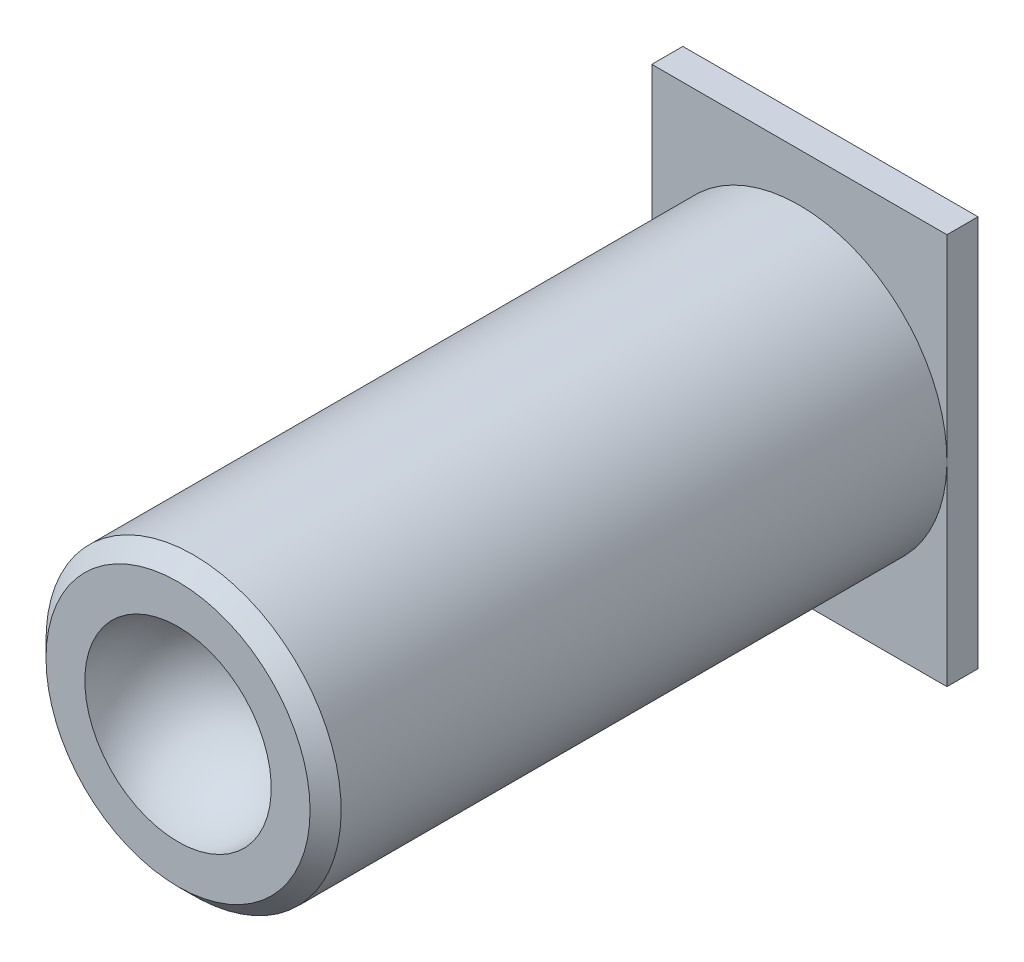
SolidWorks part; units mm, degrees
material "橡胶"
ref_plane "Front Plane" through (0, 0, 0) normal (0, 0, 1) x (1, 0, 0)
ref_plane "Top Plane" through (0, 0, 0) normal (0, 1, 0) x (1, 0, 0)
ref_plane "Right Plane" through (0, 0, 0) normal (1, 0, 0) x (0, 0, -1)
sketch "Sketch1" plane through (0, 0, 0) normal (0, 0, 1) x (1, 0, 0)
  line L0 (37, -63) -> (-37, -63) construction
  line L1 (47.5, -63) -> (-47.5, -63)
  line L2 (47.5, -63) -> (47.5, 63)
  line L3 (47.5, 63) -> (-47.5, 63)
  line L4 (-47.5, -63) -> (-47.5, 63)
  line L5 (-37, 63) -> (37, 63) construction
  line L6 (0, -63) -> (0, 63) construction
  dimension "D1" = 95
extrude "Boss-Extrude1" add sketch "Sketch1" along normal blind 10
sketch "Sketch3" plane through (0, 0, 0) normal (1, 0, 0) x (0, 0, -1)
  line L0 (-10, -63) -> (-10, 63) construction
  line L1 (-10, 0) -> (-210, 0) construction
  line L2 (-10, 0) -> (-10, 47.5)
  line L3 (-10, 47.5) -> (-205, 47.5)
  line L4 (-210, 30) -> (-210, 42.5)
  line L5 (-10, 0) -> (-180, 0)
  line L6 (-210, 42.5) -> (-205, 47.5)
  arc A0 (-180, 0) -> (-210, 30) centre (-210, 0) ccw
  point P1 (-210, 47.5)
  dimension "D2" = 30
  dimension "D1" = 200
  dimension "D3" = 47.5
revolve "Revolve1" add sketch "Sketch3" angle 360 about L1
